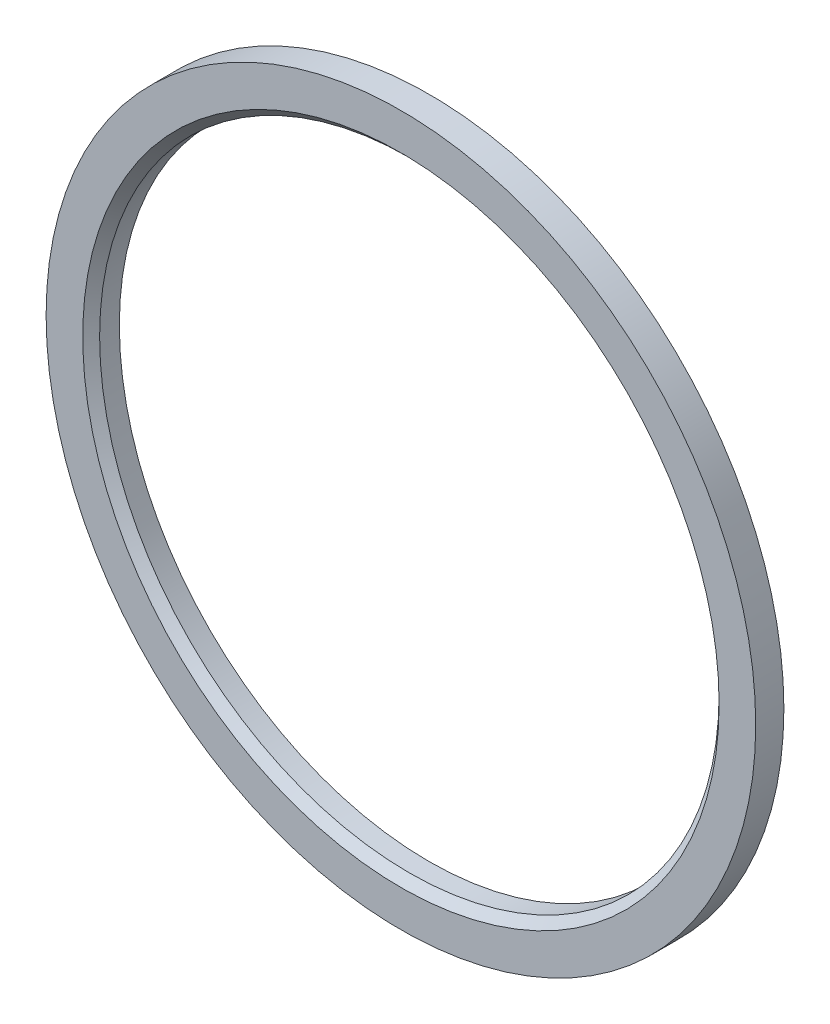
from build123d import *

# Parameters (mm, degrees)
SKETCH1_R           = 126
SKETCH1_R_2         = 110
BOSS_EXTRUDE1_DEPTH = 10
CHAMFER1_SIZE       = 3


with BuildPart() as part:
    # Sketch1 → Boss-Extrude1 (new body)
    with BuildSketch(Plane.XY):
        Circle(SKETCH1_R)
        Circle(SKETCH1_R_2, mode=Mode.SUBTRACT)
    extrude(amount=BOSS_EXTRUDE1_DEPTH)

    # Chamfer1
    chamfer1_edges = [part.edges().sort_by_distance(p)[0] for p in [
        (-110, 0, 10),
    ]]
    chamfer(chamfer1_edges, length=CHAMFER1_SIZE)


solid = part.part
